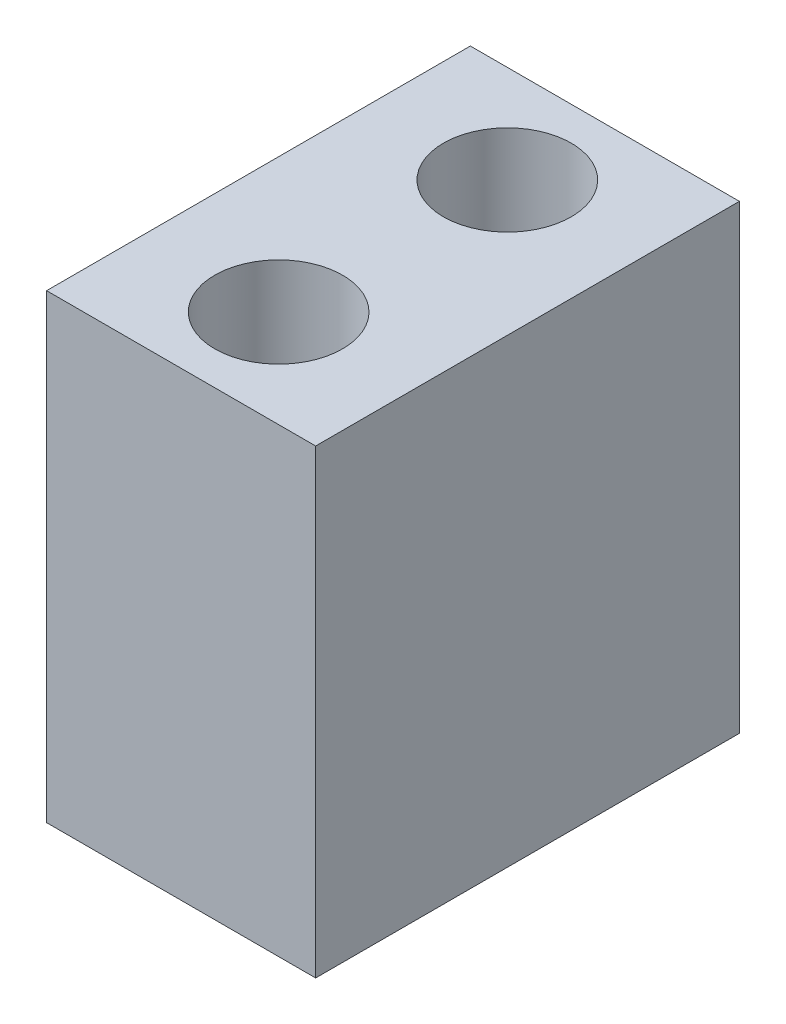
SolidWorks part; units mm, degrees
material "Q235"
ref_plane "Front Plane" through (0, 0, 0) normal (0, 0, 1) x (1, 0, 0)
ref_plane "Top Plane" through (0, 0, 0) normal (0, 1, 0) x (1, 0, 0)
ref_plane "Right Plane" through (0, 0, 0) normal (1, 0, 0) x (0, 0, -1)
sketch "Sketch2" plane through (0, 0, 0) normal (0, 1, 0) x (1, 0, 0)
  line L0 (-131.395, 0) -> (113.7022, 0) construction
  line L1 (0, 164.1787) -> (0, -121.5078) construction
  line L3 (-40, 63) -> (40, 63)
  line L4 (-40, 63) -> (-40, -63)
  line L5 (-40, -63) -> (40, -63)
  line L6 (40, 63) -> (40, -63)
  circle A0 centre (0, 34) radius 19
  circle A1 centre (0, -34) radius 19
  dimension "D5" = 38
  dimension "D1" = 126
  dimension "D2" = 80
  dimension "D3" = 40
  dimension "D4" = 68
extrude "Boss-Extrude1" add sketch "Sketch2" along normal mid plane 137
